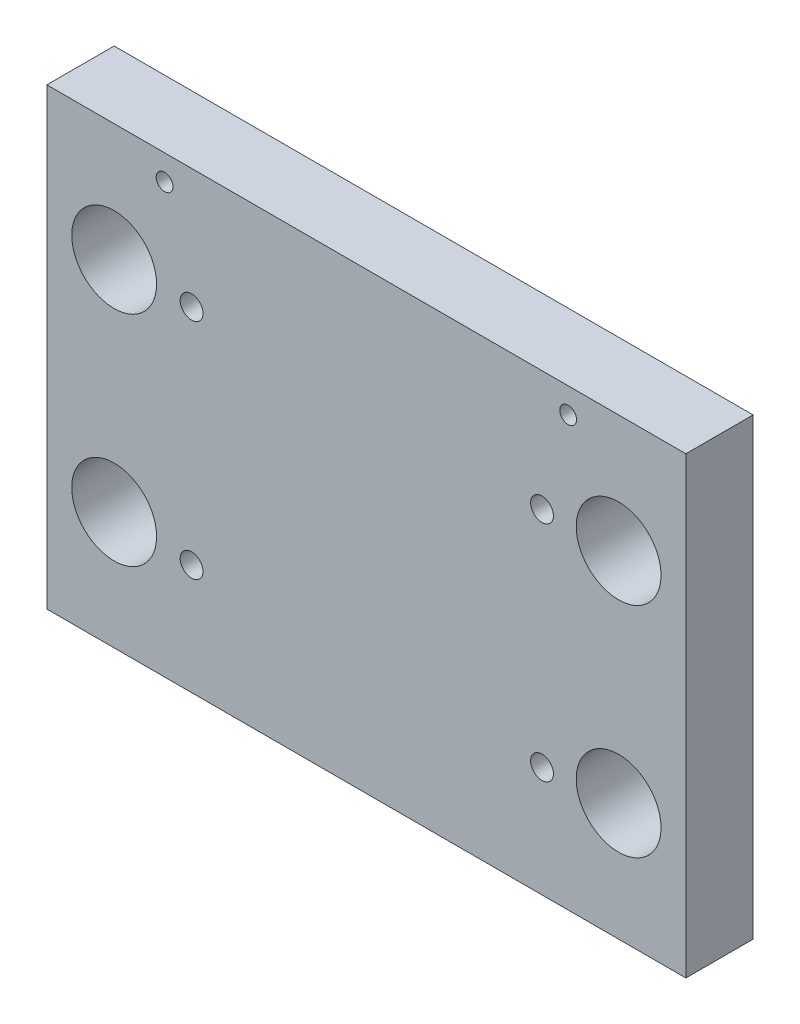
from build123d import *

# Parameters (mm, degrees)
SKETCH1_W             = 190
SKETCH1_H             = 135
SKETCH1_R             = 12.611940299
BOSS_EXTRUDE1_DEPTH   = 20
M6_TAPPED_HOLE6_D     = 5
M8_TAPPED_HOLE1_D     = 6.8
M8_TAPPED_HOLE1_DEPTH = 19.75
M8_TAPPED_HOLE1_TIP   = 2.042926105


with BuildPart() as part:
    # Sketch1 → Boss-Extrude1 (new body)
    with BuildSketch(Plane.XY):
        Rectangle(SKETCH1_W, SKETCH1_H)
        with Locations((-75, 32.5)):
            Circle(SKETCH1_R, mode=Mode.SUBTRACT)
        with Locations((-75, -32.5)):
            Circle(SKETCH1_R, mode=Mode.SUBTRACT)
        with Locations((75, 32.5)):
            Circle(SKETCH1_R, mode=Mode.SUBTRACT)
        with Locations((75, -32.5)):
            Circle(SKETCH1_R, mode=Mode.SUBTRACT)
    extrude(amount=BOSS_EXTRUDE1_DEPTH)

    # M6 Tapped Hole6 (through all)
    with Locations(Plane(origin=(0, 0, 0), x_dir=(-1, 0, 0), z_dir=(0, 0, -1))):
        with Locations((-60, 60), (60, 60)):
            Hole(M6_TAPPED_HOLE6_D / 2)

    # M8 Tapped Hole1
    with Locations(Plane.XY.offset(20)):
        with Locations((-51.96743603, 31.820881882), (-51.96743603, -34.622720538), (52.234277806, -34.622720538), (52.234277806, 31.820881882)):
            Hole(M8_TAPPED_HOLE1_D / 2, depth=M8_TAPPED_HOLE1_DEPTH)
            with Locations((0, 0, -(M8_TAPPED_HOLE1_DEPTH + M8_TAPPED_HOLE1_TIP / 2))):  # 118° drill point
                Cone(0, M8_TAPPED_HOLE1_D / 2, M8_TAPPED_HOLE1_TIP, mode=Mode.SUBTRACT)


solid = part.part
